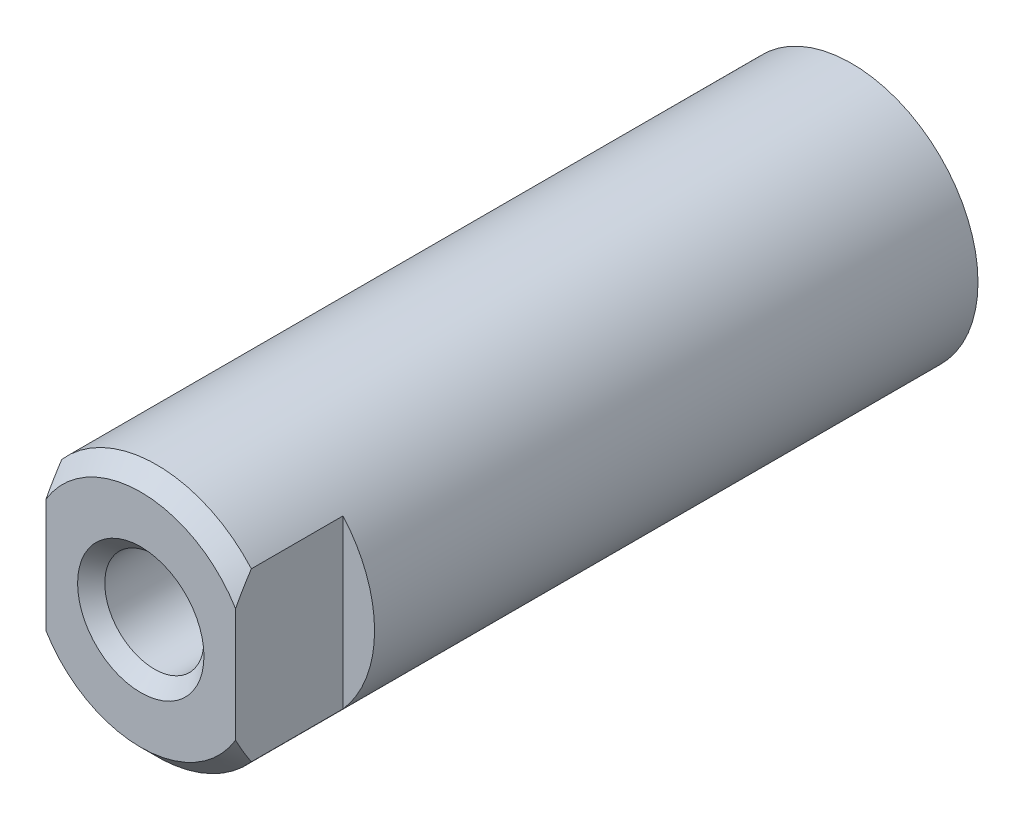
SolidWorks part; units mm, degrees
ref_plane "前视" through (0, 0, 0) normal (0, 0, 1) x (1, 0, 0)
ref_plane "上视" through (0, 0, 0) normal (0, 1, 0) x (1, 0, 0)
ref_plane "右视" through (0, 0, 0) normal (1, 0, 0) x (0, 0, -1)
sketch "草图1" plane through (0, 0, 0) normal (1, 0, 0) x (0, 0, -1)
  line L0 (-3.5, 0) -> (-3.5, 3.5)
  line L1 (-3.5, 3.5) -> (-3, 4)
  line L2 (-3, 4) -> (19, 4)
  line L3 (19, 4) -> (19, 0)
  line L4 (19, 0) -> (-3.5, 0)
  line L5 (19, 0) -> (-3.5, 0) construction
revolve "旋转1" add sketch "草图1" angle 360 about L5
ref_plane "基准面1" through (0, 0, 3.5) normal (0, 0, 1) x (1, 0, 0)
sketch "草图2" plane through (0, 0, 3.5) normal (0, 0, 1) x (1, 0, 0)
  line L0 (-6, -6) -> (-3, -6)
  line L1 (-3, -6) -> (-3, 6)
  line L2 (-3, 6) -> (3, 6)
  line L3 (3, 6) -> (3, -6)
  line L4 (3, -6) -> (6, -6)
  line L5 (6, -6) -> (6, 8)
  line L6 (6, 8) -> (-6, 8)
  line L7 (-6, 8) -> (-6, -6)
extrude "切除-拉伸1" cut sketch "草图2" against normal blind 3.4
sketch "草图3" plane through (0, 0, 0) normal (1, 0, 0) x (0, 0, -1)
  line L0 (-4, 0) -> (-4, 2.5)
  line L1 (-4, 2.5) -> (-3.07, 1.57)
  line L2 (-3.07, 1.57) -> (5, 1.57)
  line L3 (5, 1.57) -> (5.9064, 0)
  line L4 (5.9064, 0) -> (-4, 0)
  line L5 (5.9064, 0) -> (-4, 0) construction
revolve "切除-旋转1" cut sketch "草图3" angle 360 about L5
ref_plane "基准面2" through (0, 0, 3.5) normal (0, 0, 1) x (1, 0, 0)
